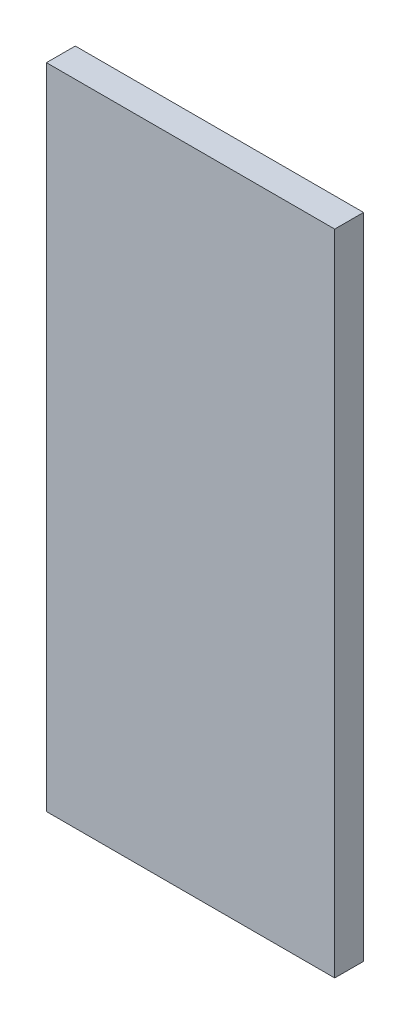
SolidWorks part; units mm, degrees
ref_plane "前视基准面" through (0, 0, 0) normal (0, 0, 1) x (1, 0, 0)
ref_plane "上视基准面" through (0, 0, 0) normal (0, 1, 0) x (1, 0, 0)
ref_plane "右视基准面" through (0, 0, 0) normal (1, 0, 0) x (0, 0, -1)
sketch "草图1" plane through (0, 0, 0) normal (0, 0, 1) x (1, 0, 0)
  line L0 (0, 0) -> (80, 0)
  line L1 (80, 0) -> (80, 180)
  line L2 (80, 180) -> (0, 180)
  line L3 (0, 180) -> (0, 0)
extrude "凸台-拉伸1" add sketch "草图1" against normal blind 8
